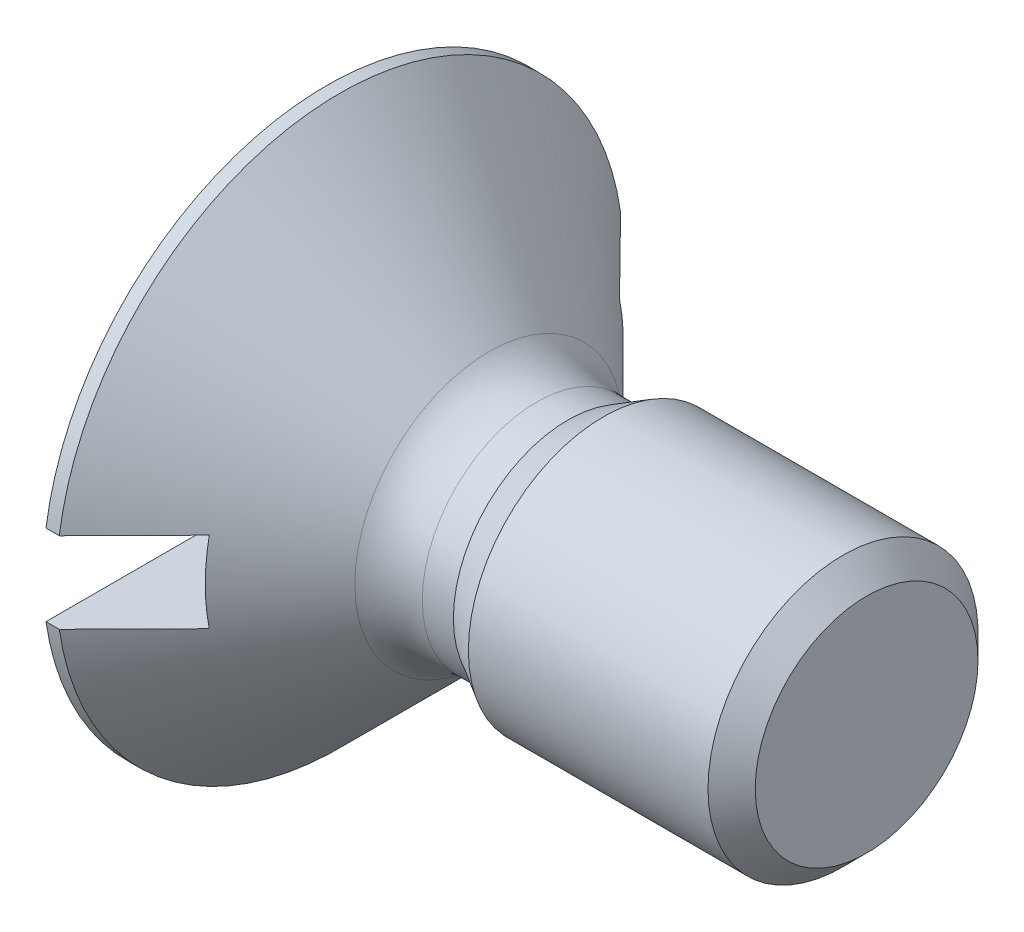
SolidWorks part; units mm, degrees
ref_plane "Front Plane" through (0, 0, 0) normal (0, 0, 1) x (1, 0, 0)
ref_plane "Top Plane" through (0, 0, 0) normal (0, 1, 0) x (1, 0, 0)
ref_plane "Right Plane" through (0, 0, 0) normal (1, 0, 0) x (0, 0, -1)
sketch "Dimension Sketch" plane through (0, 0, 0) normal (0, 0, 1) x (1, 0, 0)
  line L0 (0, 0) -> (8, 0) construction
  point P3 (4, 0)
  point P4 (8.4, 0)
  point P5 (0.7, 0)
  point P6 (1.4, 0)
  point P7 (1.2, 0)
  point P8 (1, 0)
  point P9 (2.7, 0)
  point P10 (6.7, 0)
  dimension "l" = 8
  dimension "d" = 4
  dimension "dk" = 8.4
  dimension "p" = 0.7
  dimension "a" = 1.4
  dimension "k" = 2.7
  dimension "n" = 1.2
  dimension "r" = 1
  dimension "t" = 1.3
sketch "Sketch1" plane through (0, 0, 0) normal (0, 0, 1) x (1, 0, 0)
  line L0 (0, 0) -> (128.7124, 0) construction
  line L1 (0, 0) -> (0, 4.2)
  line L2 (0, 4.2) -> (0.1969, 4.2)
  line L3 (0.1969, 4.2) -> (2.4071, 1.9898)
  line L4 (3.1142, 1.6969) -> (3.575, 1.6969)
  line L5 (3.575, 1.6969) -> (4.1, 2)
  line L6 (4.1, 2) -> (8, 2)
  line L7 (8, 2) -> (8, 0)
  line L8 (0, 0) -> (8, 0)
  arc A0 (3.1142, 1.6969) -> (2.4071, 1.9898) centre (3.1142, 2.6969) cw
  point P12 (2.7, 1.6969)
  dimension "r" = 1
  dimension "D1" = 45
  dimension "D2" = 30
  dimension "D3" = 3.3938
  dimension "k" = 2.7
  dimension "d" = 4
  dimension "dk" = 8.4
  dimension "a" = 1.4
  dimension "l" = 8
revolve "Base-Revolve" add sketch "Sketch1" angle 360 about L0
cosmetic thread "Cosmetic Thread1" parameters "D2"=3.3938
chamfer "Chamfer1" distance 0.35 angle 45 1 edges at (8, 0, 2)
sketch "Sketch3" plane through (0, 0, 0) normal (-1, 0, 0) x (0, 0, 1)
  line L0 (0, 0) -> (1.6419, 0) construction
  line L2 (-4.1569, 0.6) -> (4.1569, 0.6)
  line L4 (-4.1569, -0.6) -> (4.1569, -0.6)
  arc A0 (4.1569, -0.6) -> (4.1569, 0.6) centre (0, 0) ccw
  circle A1 centre (0, 0) radius 4.2
  arc A2 (-4.1569, 0.6) -> (-4.1569, -0.6) centre (0, 0) ccw
  dimension "n" = 1.2
  dimension "D1" = 0
extrude "Cut-Extrude1" cut sketch "Sketch3" against normal blind 1.3
sketch "Sketch2" plane through (0, 0, 0) normal (0, 0, 1) x (1, 0, 0)
  line L0 (7.65, 2) -> (8.35, 2)
  line L1 (8.35, 2) -> (8, 1.3938)
  line L2 (8, 1.3938) -> (7.65, 2)
  line L3 (8, 2) -> (8, 1.3938) construction
  line L6 (8, -1.65) -> (8, 1.65) construction
  line L8 (0, 0) -> (128.7124, 0) construction
  line L9 (3.3795, 0) -> (4.4719, 0) construction
  dimension "D1" = 2
  dimension "p" = 0.7
revolve "Cut-Revolve1" [suppressed] cut sketch "Sketch2" angle 360 about L9
pattern_linear "LPattern1" [suppressed] count 6 spacing 0.7 along (1, 0, 0)
